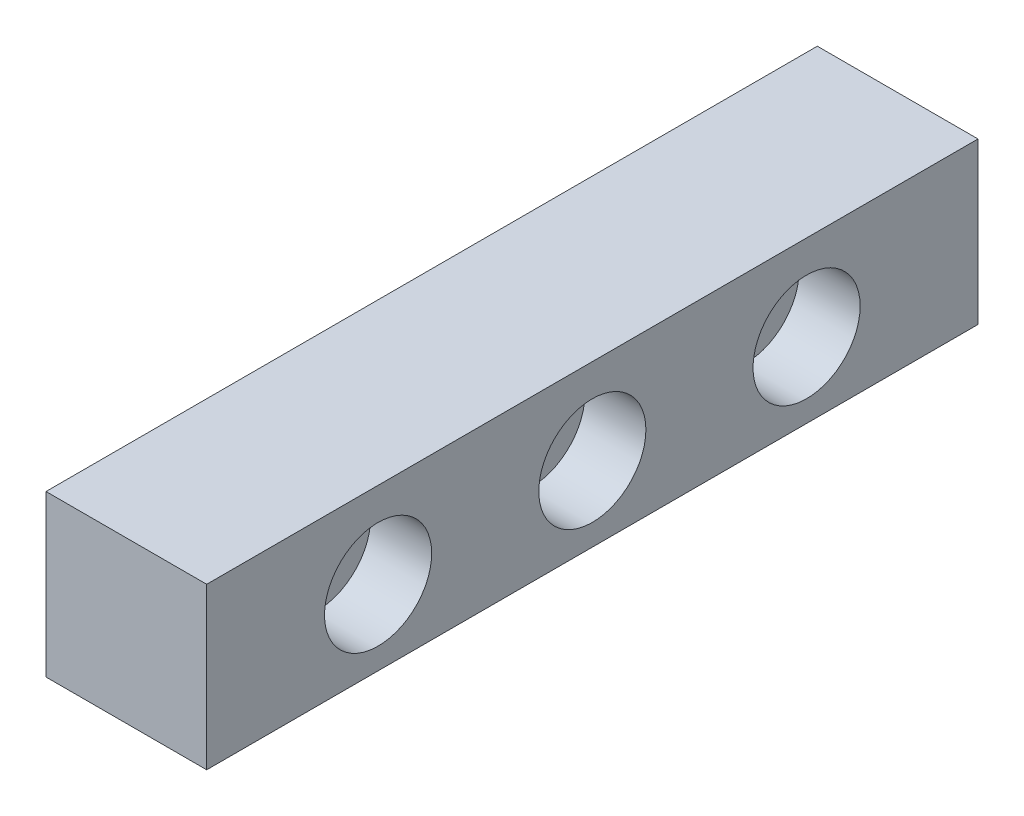
SolidWorks part; units mm, degrees
ref_plane "前视基准面" through (0, 0, 0) normal (0, 0, 1) x (1, 0, 0)
ref_plane "上视基准面" through (0, 0, 0) normal (0, 1, 0) x (1, 0, 0)
ref_plane "右视基准面" through (0, 0, 0) normal (1, 0, 0) x (0, 0, -1)
sketch "草图1" plane through (0, 0, 0) normal (1, 0, 0) x (0, 0, -1)
  line L1 (-36, 7.5) -> (36, 7.5)
  line L2 (-36, 7.5) -> (-36, -7.5)
  line L3 (-36, -7.5) -> (36, -7.5)
  line L4 (36, 7.5) -> (36, -7.5)
  line L5 (-36, 7.5) -> (36, -7.5) construction
  line L6 (-36, -7.5) -> (36, 7.5) construction
  point P0 (0, 0)
  dimension "D1" = 72
  dimension "D2" = 15
extrude "凸台-拉伸1" add sketch "草图1" along normal blind 15
hole_wizard "打孔尺寸(%根据)内六角圆柱头螺钉的类型2" positions "草图2" profile "草图3" counterbore size "M5" standard "GB" end condition through all
sketch "草图2" plane through (15, 0, 0) normal (1, 0, 0) x (0, 0, -1)
  line L0 (0, -7.5) -> (0, 14.364) construction
  line L1 (-36, -7.5) -> (36, -7.5) construction
  line L3 (36, 7.5) -> (-36, 7.5) construction
  point P0 (-20, -0.5)
  point P2 (0, -0.5)
  point P5 (20, -0.5)
  dimension "D1" = 40
  dimension "D2" = 8
sketch "草图3" plane through (15, -0.5, 20) normal (0, 1, 0) x (0, 0, -1)
  line L0 (0, 0) -> (0, 15)
  line L1 (0, 15) -> (2.75, 15)
  line L3 (2.75, 15) -> (2.75, 5.7)
  line L4 (2.75, 5.7) -> (5, 5.7)
  line L5 (5, 5.7) -> (5, 0)
  line L7 (5, 0) -> (0, 0)
  line L11 (0, -6.35) -> (0, 107.95) construction
  dimension "通孔孔直径" = 5.5
  dimension "通孔孔深度" = 15
  dimension "柱形沉头孔直径" = 10
  dimension "柱形沉头孔深度" = 5.7
